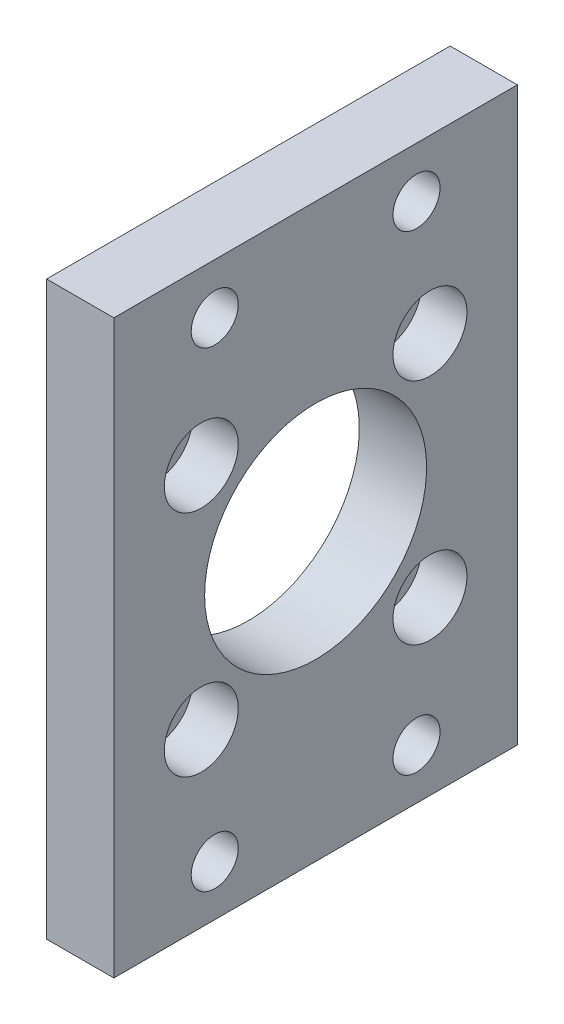
SolidWorks part; units mm, degrees
ref_plane "前视基准面" through (0, 0, 0) normal (0, 0, 1) x (1, 0, 0)
ref_plane "上视基准面" through (0, 0, 0) normal (0, 1, 0) x (1, 0, 0)
ref_plane "右视基准面" through (0, 0, 0) normal (1, 0, 0) x (0, 0, -1)
sketch "草图1" plane through (0, 0, 0) normal (1, 0, 0) x (0, 0, -1)
  line L1 (-30, 42.5) -> (30, 42.5)
  line L2 (-30, 42.5) -> (-30, -42.5)
  line L3 (-30, -42.5) -> (30, -42.5)
  line L4 (30, 42.5) -> (30, -42.5)
  line L5 (-30, 42.5) -> (30, -42.5) construction
  line L6 (-30, -42.5) -> (30, 42.5) construction
  point P0 (0, 0)
  dimension "D1" = 60
  dimension "D2" = 85
extrude "凸台-拉伸1" add sketch "草图1" along normal blind 10
hole_wizard "打孔尺寸(%根据)内六角圆柱头螺钉的类型1" positions "草图2" profile "草图3" counterbore size "M6" standard "GB" end condition through all
sketch "草图2" plane through (10, 0, 0) normal (1, 0, 0) x (0, 0, -1)
  line L0 (0, 51.8216) -> (0, -43.7455) construction
  line L2 (-42.4836, 0) -> (72.769, 0) construction
  point P0 (-17, 17)
  point P2 (17, 17)
  point P4 (-17, -17)
  point P6 (17, -17)
  dimension "D1" = 34
  dimension "D2" = 34
sketch "草图3" plane through (10, 17, 17) normal (0, 1, 0) x (0, 0, -1)
  line L0 (0, 0) -> (0, 10)
  line L1 (0, 10) -> (3.3, 10)
  line L3 (3.3, 10) -> (3.3, 6.8)
  line L4 (3.3, 6.8) -> (5.5, 6.8)
  line L5 (5.5, 6.8) -> (5.5, 0)
  line L7 (5.5, 0) -> (0, 0)
  line L11 (0, -6.35) -> (0, 107.95) construction
  dimension "通孔孔直径" = 6.6
  dimension "通孔孔深度" = 10
  dimension "柱形沉头孔直径" = 11
  dimension "柱形沉头孔深度" = 6.8
hole_wizard "Ø7.0 (7) 直径孔1" positions "草图4" profile "草图5" hole size "Ø7.0" standard "GB" end condition through all
sketch "草图4" plane through (0, 0, 0) normal (-1, 0, 0) x (0, 0, 1)
  line L0 (0, 76.7552) -> (0, -63.0905) construction
  line L2 (-48.6989, 0) -> (70.5043, 0) construction
  point P0 (-15, 35)
  point P2 (15, 35)
  point P4 (-15, -35)
  point P6 (15, -35)
  dimension "D1" = 30
  dimension "D2" = 70
sketch "草图5" plane through (0, 35, -15) normal (0, 1, 0) x (0, 0, 1)
  line L0 (0, 0) -> (0, 10)
  line L1 (0, 10) -> (3.5, 10)
  line L2 (3.5, 10) -> (3.5, 0)
  line L5 (3.5, 0) -> (0, 0)
  line L11 (0, -6.35) -> (0, 107.95) construction
  dimension "通孔孔直径" = 7
  dimension "通孔孔深度" = 10
sketch "草图6" plane through (0, 0, 0) normal (-1, 0, 0) x (0, 0, 1)
  circle A0 centre (0, 0) radius 16.5
  dimension "D1" = 33
extrude "切除-拉伸1" cut sketch "草图6" against normal through all
